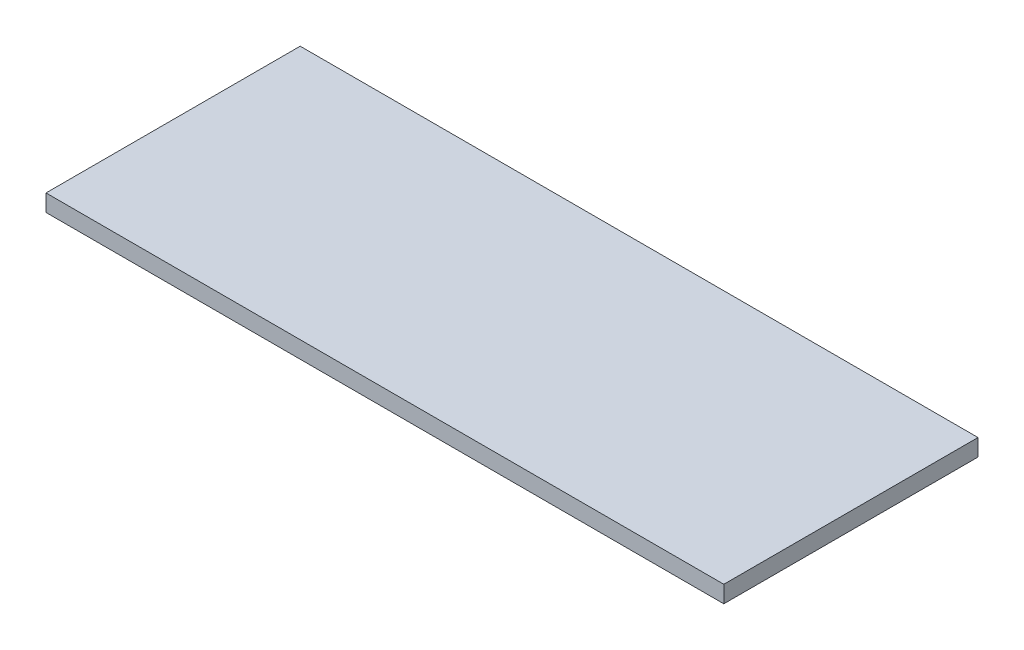
SolidWorks part; units mm, degrees
ref_plane "前视基准面" through (0, 0, 0) normal (0, 0, 1) x (1, 0, 0)
ref_plane "上视基准面" through (0, 0, 0) normal (0, 1, 0) x (1, 0, 0)
ref_plane "右视基准面" through (0, 0, 0) normal (1, 0, 0) x (0, 0, -1)
sketch "草图1" plane through (0, 0, 0) normal (0, 1, 0) x (1, 0, 0)
  line L1 (-20, -7.5) -> (20, -7.5)
  line L2 (-20, -7.5) -> (-20, 7.5)
  line L3 (-20, 7.5) -> (20, 7.5)
  line L4 (20, -7.5) -> (20, 7.5)
  line L5 (-20, -7.5) -> (20, 7.5) construction
  line L6 (-20, 7.5) -> (20, -7.5) construction
  point P0 (0, 0)
  dimension "D1" = 40
  dimension "D2" = 15
extrude "凸台-拉伸1" add sketch "草图1" along normal blind 1
